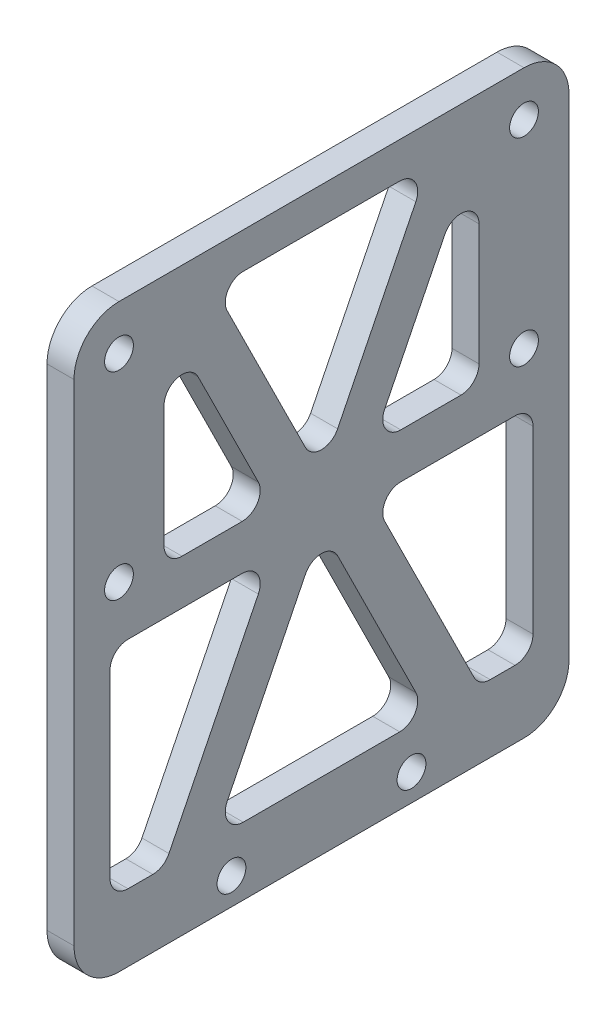
SolidWorks part; units mm, degrees
material "哈碳纤"
ref_plane "前视基准面" through (0, 0, 0) normal (0, 0, 1) x (1, 0, 0)
ref_plane "上视基准面" through (0, 0, 0) normal (0, 1, 0) x (1, 0, 0)
ref_plane "右视基准面" through (0, 0, 0) normal (1, 0, 0) x (0, 0, -1)
other "Configuration Table"
sketch "草图2" plane through (0, 0, 0) normal (1, 0, 0) x (0, 0, -1)
  line L1 (0, 0) -> (55, 0)
  line L2 (0, 0) -> (0, 64.5)
  line L3 (0, 64.5) -> (55, 64.5)
  line L4 (55, 0) -> (55, 64.5)
  dimension "D1" = 64.5
  dimension "D2" = 55
extrude "凸台-拉伸1" add sketch "草图2" along normal blind 3
sketch "草图3" plane through (0, 0, 0) normal (-1, 0, 0) x (0, 0, 1)
  line L0 (-55, 64.5) -> (0, 64.5) construction
  line L1 (-50, 37.5) -> (-5, 37.5) construction
  line L2 (-50, 37.5) -> (-50, 59.5) construction
  line L3 (-50, 59.5) -> (-5, 59.5) construction
  line L4 (-5, 37.5) -> (-5, 59.5) construction
  line L6 (-27.5, 64.5) -> (-27.5, 0) construction
  line L7 (0, 0) -> (-55, 0) construction
  line L9 (-37.5, 3) -> (-17.5, 3) construction
  circle A0 centre (-5, 59.5) radius 1.6
  circle A1 centre (-5, 37.5) radius 1.6
  circle A2 centre (-50, 59.5) radius 1.6
  circle A3 centre (-50, 37.5) radius 1.6
  circle A4 centre (-37.5, 3) radius 1.6
  circle A5 centre (-17.5, 3) radius 1.6
  point P14 (-27.5, 59.5)
  point P19 (-27.5, 3)
  dimension "D3" = 3.2
  dimension "D4" = 3.2
  dimension "D5" = 3.2
  dimension "D6" = 3.2
  dimension "D8" = 3.2
  dimension "D9" = 3.2
  dimension "D1" = 22
  dimension "D2" = 45
  dimension "D7" = 5
  dimension "D10" = 20
  dimension "D11" = 3
extrude "切除-拉伸1" cut sketch "草图3" against normal blind 3
fillet "圆角1" radius 5 4 edges at (1.5, 64.5, 0) (1.5, 64.5, -55) (1.5, 0, 0) (1.5, 0, -55)
sketch "草图4" plane through (0, 0, 0) normal (-1, 0, 0) x (0, 0, 1)
  line L0 (-39.4175, 60.5) -> (-27.5, 36.5)
  line L1 (-15.5825, 60.5) -> (-27.5, 36.5)
  line L2 (-39.4175, 60.5) -> (-15.5825, 60.5)
  line L3 (-1027.5, 34) -> (48972.5, 34) construction
  line L4 (-27.5, 4.432) -> (-27.5, 49000) construction
  line L5 (-5, 0) -> (-50, 0) construction
  line L6 (-45, 60.5) -> (-45, 36.5)
  line L7 (-45, 36.5) -> (-33.0825, 36.5)
  line L8 (-33.0825, 36.5) -> (-45, 60.5)
  line L9 (-21.9175, 36.5) -> (-10, 60.5)
  line L10 (-10, 36.5) -> (-21.9175, 36.5)
  line L11 (-10, 60.5) -> (-10, 36.5)
  line L12 (972.5, 34) -> (-49027.5, 34) construction
  line L13 (-50, 64.5) -> (-5, 64.5) construction
  line L14 (0, 59.5) -> (0, 5) construction
  line L15 (-10, 31.5) -> (-21.9175, 31.5)
  line L17 (-21.9175, 31.5) -> (-10, 7.5)
  line L18 (-39.4175, 7.5) -> (-27.5, 31.5)
  line L19 (-15.5825, 7.5) -> (-27.5, 31.5)
  line L21 (-45, 31.5) -> (-33.0825, 31.5)
  line L23 (-33.0825, 31.5) -> (-45, 7.5)
  line L24 (-39.4175, 7.5) -> (-15.5825, 7.5)
  line L25 (-45, 31.5) -> (-51, 31.5)
  line L26 (-51, 31.5) -> (-51, 7.5)
  line L27 (-51, 7.5) -> (-45, 7.5)
  line L28 (-10, 31.5) -> (-4, 31.5)
  line L29 (-4, 7.5) -> (-10, 7.5)
  line L30 (-4, 31.5) -> (-4, 7.5)
  line L31 (-55, 5) -> (-55, 59.5) construction
  point P5 (-27.5, 0)
  point P9 (-27.5, 60.5)
  dimension "D1" = 24
  dimension "D2" = 5
  dimension "D3" = 2.5
  dimension "D4" = 4
  dimension "D5" = 10
  dimension "D6" = 4
  dimension "D7" = 7.5
extrude "切除-拉伸2" cut sketch "草图4" against normal blind 3
fillet "圆角2" radius 2 20 edges at (1.5, 7.5, -10) (1.5, 31.5, -21.9175) (1.5, 31.5, -4) (1.5, 7.5, -4) (1.5, 7.5, -39.4175) (1.5, 31.5, -27.5) (1.5, 7.5, -15.5825) (1.5, 36.5, -27.5) (1.5, 60.5, -39.4175) (1.5, 60.5, -15.5825) (1.5, 36.5, -45) (1.5, 36.5, -33.0825) (1.5, 60.5, -10) (1.5, 36.5, -10) (1.5, 36.5, -21.9175) (1.5, 31.5, -33.0825) (1.5, 7.5, -45) (1.5, 7.5, -51) (1.5, 31.5, -51) (1.5, 60.5, -45)
